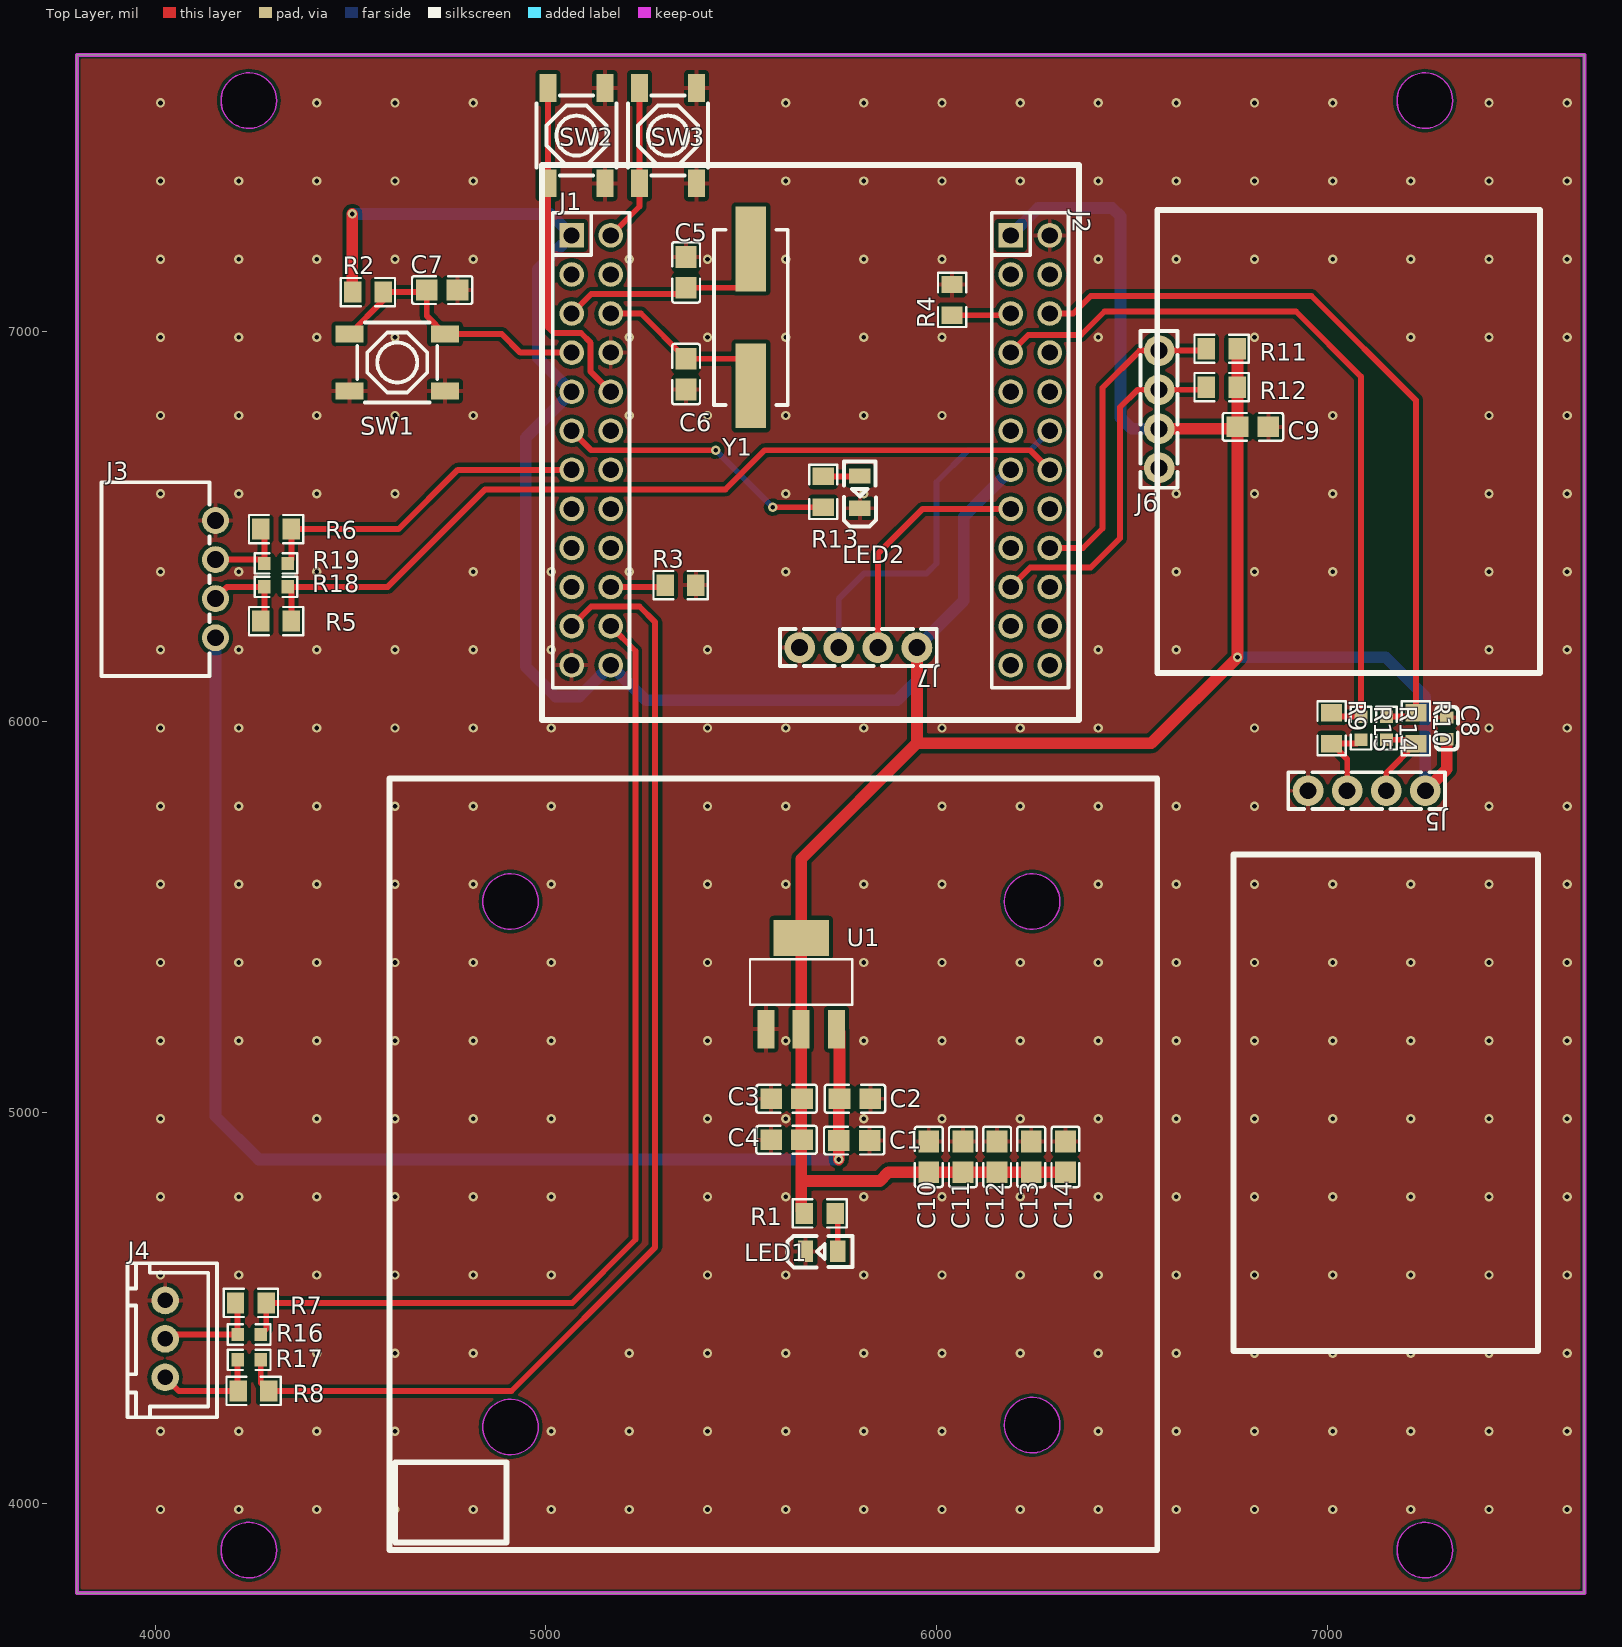
[diagram p0: Top Layer view]
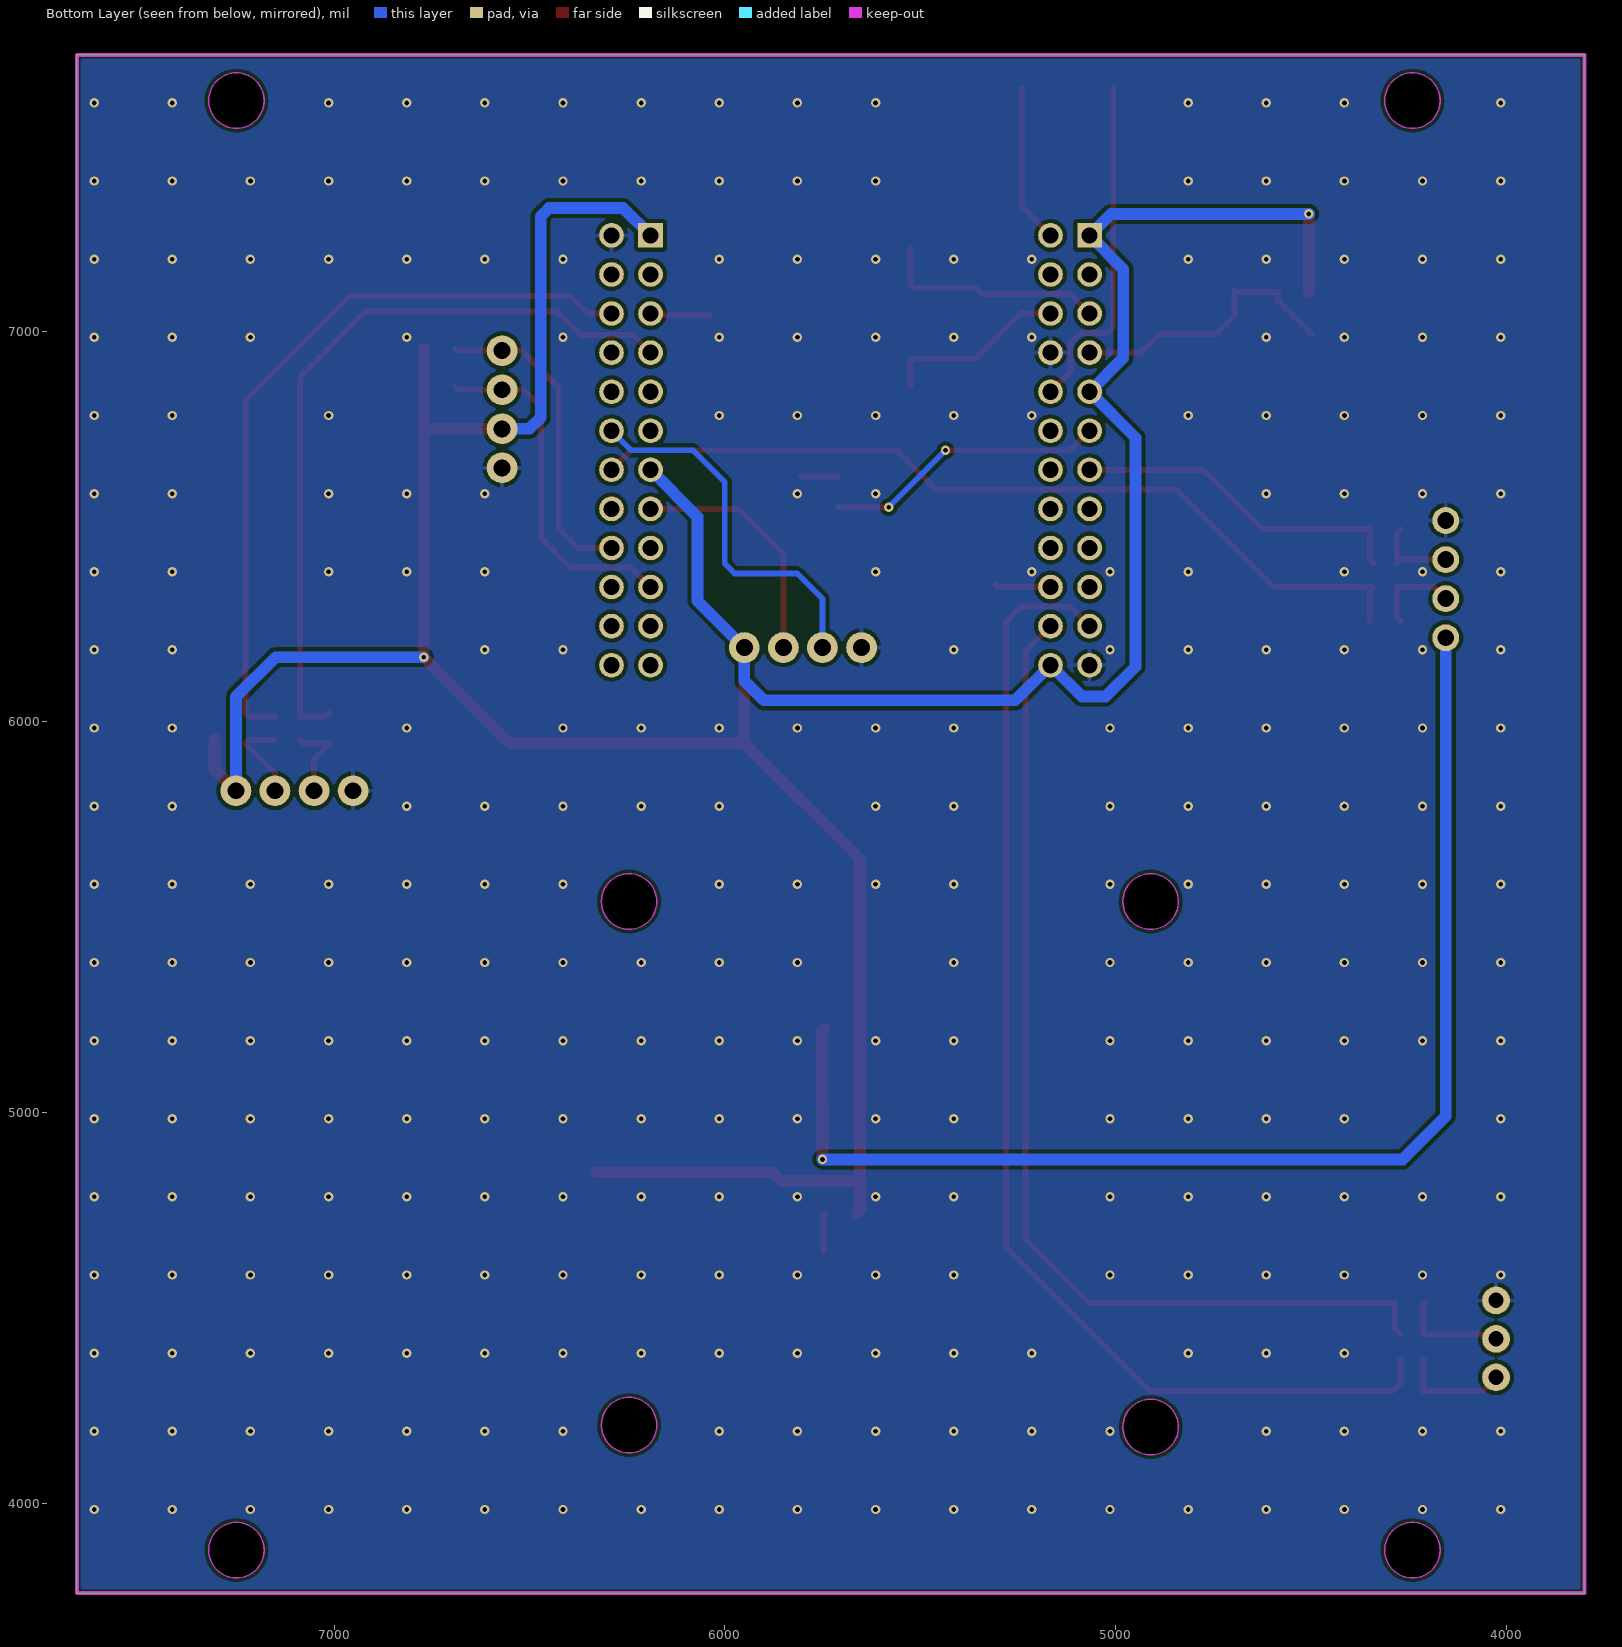
[diagram p1: Bottom Layer view, seen from below]
# Altium PCB MISC52078.pcbdoc
Units mil, origin at the board's own origin, x right, y up, seen from the top; angles counter-clockwise.
Board outline 3858.27 x 3937.01 mil, 2 copper layers (Top Layer, Bottom Layer), stack 2.757 mil thick; 47 components, 30 nets, 155 pads, 300 vias.

## Layer stack, top to bottom
Top Solder Mask Layer: solder mask 0.394, Dk 3.3
Top Layer: signal copper 1.379
Bottom Layer: signal copper 1.378
Bottom Solder Mask Layer: solder mask 0.394, Dk 3.3

## Board outline
3800,7707.01 3800,3770 7658.27,3770 7658.27,7707.01
cut-out: 4981.06,5540 cw(c4910,5540) 4838.94,5540 cw(c4910,5540)
cut-out: 6316.06,5540 cw(c6245,5540) 6173.94,5540 cw(c6245,5540)
cut-out: 6316.06,4200 cw(c6245,4200) 6173.94,4200 cw(c6245,4200)
cut-out: 4981.06,4195 cw(c4910,4195) 4838.94,4195 cw(c4910,4195)
cut-out: 4311.06,3880 cw(c4240,3880) 4168.94,3880 cw(c4240,3880)
cut-out: 4311.06,7590 cw(c4240,7590) 4168.94,7590 cw(c4240,7590)
cut-out: 7321.06,7590 cw(c7250,7590) 7178.94,7590 cw(c7250,7590)
cut-out: 7321.06,3880 cw(c7250,3880) 7178.94,3880 cw(c7250,3880)

## Design rules (kind name [scope] priority, off if disabled: settings)
BoardOutlineClearance Plane_innerPlane_1 [All] p2 off: genericclearance=4 ignorepadtopadclearanceinfootprint=FALSE except(0: Arc-SplitContinuation Track-SplitContinuation SMDPad-SplitContinuation THPad-SplitContinuation Via-SplitContinuation Fill-SplitContinuation Region-SplitContinuation Poly-SplitContinuation Text-SplitContinuation Hole-SplitContinuation; 6: Arc-CutoutEdge Track-CutoutEdge SMDPad-CutoutEdge THPad-CutoutEdge Via-CutoutEdge Text-CutoutEdge; 6.9: Hole-OutlineEdge Hole-CutoutEdge; 10: Poly-OutlineEdge Poly-CutoutEdge; 11.8: Arc-OutlineEdge Track-OutlineEdge SMDPad-OutlineEdge THPad-OutlineEdge Via-OutlineEdge Fill-OutlineEdge Region-OutlineEdge Text-OutlineEdge Fill-CutoutEdge Region-CutoutEdge)
BoardOutlineClearance Copper_copperRegion_1 [All] p4 off: genericclearance=4 ignorepadtopadclearanceinfootprint=FALSE except(0: Arc-SplitContinuation Track-SplitContinuation SMDPad-SplitContinuation THPad-SplitContinuation Via-SplitContinuation Fill-SplitContinuation Region-SplitContinuation Poly-SplitContinuation Text-SplitContinuation Hole-SplitContinuation; 6: Arc-CutoutEdge Track-CutoutEdge SMDPad-CutoutEdge THPad-CutoutEdge Via-CutoutEdge Text-CutoutEdge; 6.9: Hole-OutlineEdge Hole-CutoutEdge; 10: Poly-OutlineEdge Poly-CutoutEdge; 11.8: Arc-OutlineEdge Track-OutlineEdge SMDPad-OutlineEdge THPad-OutlineEdge Via-OutlineEdge Fill-OutlineEdge Region-OutlineEdge Text-OutlineEdge Fill-CutoutEdge Region-CutoutEdge)
BoardOutlineClearance copperThickness1oz_1 [All] p6: genericclearance=4 ignorepadtopadclearanceinfootprint=FALSE except(0: Arc-SplitContinuation Track-SplitContinuation SMDPad-SplitContinuation THPad-SplitContinuation Via-SplitContinuation Fill-SplitContinuation Region-SplitContinuation Poly-SplitContinuation Text-SplitContinuation Hole-SplitContinuation; 6: Arc-CutoutEdge Track-CutoutEdge SMDPad-CutoutEdge THPad-CutoutEdge Via-CutoutEdge Text-CutoutEdge; 6.9: Hole-OutlineEdge Hole-CutoutEdge; 10: Poly-OutlineEdge Poly-CutoutEdge; 11.8: Arc-OutlineEdge Track-OutlineEdge SMDPad-OutlineEdge THPad-OutlineEdge Via-OutlineEdge Fill-OutlineEdge Region-OutlineEdge Text-OutlineEdge Fill-CutoutEdge Region-CutoutEdge)
Clearance Plane_innerPlane [All] p1 off: gap=4 ignorepadtopadclearanceinfootprint=FALSE except(6: SMDPad-Track SMDPad-SMDPad THPad-Track SMDPad-THPad THPad-THPad Track-Via SMDPad-Via THPad-Via Via-Via Fill-SMDPad Region-SMDPad Fill-THPad Region-THPad Fill-Via Region-Via Fill-Fill Fill-Region Region-Region Arc-Track Arc-SMDPad Arc-THPad Arc-Via Fill-Arc Region-Arc Arc-Arc Text-Track SMDPad-Text Text-THPad Text-Via Fill-Text Region-Text Arc-Text Text-Text; 6.9: Hole-Track Hole-SMDPad Hole-THPad Hole-Via Fill-Hole Region-Hole Hole-Arc Hole-Text; 10: Poly-Track Poly-SMDPad Poly-THPad Poly-Via Poly-Fill Poly-Region Poly-Poly Poly-Arc Poly-Text Poly-Hole; 11.8: Fill-Track Region-Track)
Clearance Copper_copperRegion [All] p3 off: gap=4 ignorepadtopadclearanceinfootprint=FALSE except(6: SMDPad-Track SMDPad-SMDPad THPad-Track SMDPad-THPad THPad-THPad Track-Via SMDPad-Via THPad-Via Via-Via Fill-SMDPad Region-SMDPad Fill-THPad Region-THPad Fill-Via Region-Via Fill-Fill Fill-Region Region-Region Arc-Track Arc-SMDPad Arc-THPad Arc-Via Fill-Arc Region-Arc Arc-Arc Text-Track SMDPad-Text Text-THPad Text-Via Fill-Text Region-Text Arc-Text Text-Text; 6.9: Hole-Track Hole-SMDPad Hole-THPad Hole-Via Fill-Hole Region-Hole Hole-Arc Hole-Text; 10: Poly-Track Poly-SMDPad Poly-THPad Poly-Via Poly-Fill Poly-Region Poly-Poly Poly-Arc Poly-Text Poly-Hole; 11.8: Fill-Track Region-Track)
Clearance copperThickness1oz [All] p5: gap=4 ignorepadtopadclearanceinfootprint=FALSE except(6: SMDPad-Track SMDPad-SMDPad THPad-Track SMDPad-THPad THPad-THPad Track-Via SMDPad-Via THPad-Via Via-Via Fill-SMDPad Region-SMDPad Fill-THPad Region-THPad Fill-Via Region-Via Fill-Fill Fill-Region Region-Region Arc-Track Arc-SMDPad Arc-THPad Arc-Via Fill-Arc Region-Arc Arc-Arc Text-Track SMDPad-Text Text-THPad Text-Via Fill-Text Region-Text Arc-Text Text-Text; 6.9: Hole-Track Hole-SMDPad Hole-THPad Hole-Via Fill-Hole Region-Hole Hole-Arc Hole-Text; 10: Poly-Track Poly-SMDPad Poly-THPad Poly-Via Poly-Fill Poly-Region Poly-Poly Poly-Arc Poly-Text Poly-Hole; 11.8: Fill-Track Region-Track)
DiffPairsRouting differentialPair [All] p1: maxlimit=6 minlimit=5 mostfreqgap=6 toplayer_minwidth=5 toplayer_prefwidth=100 toplayer_maxwidth=100 toplayer_mingap=5 toplayer_prefgap=6 toplayer_maxgap=6 bottomlayer_minwidth=5 bottomlayer_prefwidth=100 bottomlayer_maxwidth=100 bottomlayer_mingap=5 bottomlayer_prefgap=6 bottomlayer_maxgap=6 maxuncoupledlength=10
HoleToHoleClearance otherClearance [All] p1: gap=11.8 allowstackedmicrovias=TRUE
Length netLength [All] p1: minlimit=0 maxlimit=0
MatchedLengths netLengthTolerance [All] p1: tolerance=1000
PasteMaskExpansion pasteMaskExpansion [All] p1: expansion=0
PlaneConnect innerPlane [All] p1: planeconnectstyle=Relief reliefexpansion=20 reliefentries=4 reliefconductorwidth=10 reliefairgap=10
PolygonConnect copperRegion [(InNet('GND'))] p1: connectstyle=Relief reliefconductorwidth=10 reliefentries=4 polygonreliefangle="90 Angle" airgapwidth=10 via.connectstyle=Relief via.reliefconductorwidth=10 via.reliefentries=4 via.polygonreliefangle="90 Angle" via.airgapwidth=10
RoutingVias viaSize [All] p1: holewidth=12.01 width=24.02 viastyle="Through Hole" minholewidth=11.81 minwidth=19.68 maxholewidth=248.03 maxwidth=393.7
SolderMaskExpansion solderMaskExpansion [IsVia] p1: expansion=-1000 istentingtop=TRUE
SolderMaskExpansion solderMaskExpansion [All] p2: expansion=2 istentingtop=FALSE
Width copperThickness1oz_2 [All] p1: maxlimit=100 minlimit=5 preferedwidth=10

## Components (designator, comment, footprint, x,y, rotation, side; value= is the part's Value field where it differs from the comment)
C1 "10uF" C0805 5789.54,4928.26 r0 top
C2 "0.1uF" C0805 5791.42,5035.2 r0 top
C3 "10uF" C0805 5616.42,5035.2 r0 top
C4 "0.1uF" C0805 5616.42,4930.2 r0 top
C5 "20pF" C0805 5359.24,7150.22 r270 top
C6 "20pF" C0805 5359.24,6890 r90 top
C7 "10uF" C0805 4735,7105 r0 top
C8 "0.1uF" C0603 7306.26,5983.34 r270 top
C9 "0.1uF" C0805 6810,6755 r0 top
C10 "0.1uF" C0805 5980.2,4886.53 r90 top
C11 "0.1uF" C0805 6067.7,4886.53 r90 top
C12 "0.1uF" C0805 6155.2,4886.53 r90 top
C13 "0.1uF" C0805 6242.7,4886.53 r90 top
C14 "0.1uF" C0805 6330.2,4886.53 r90 top
J1 "PM254-2-12-Z-8.5" HDR-TH_24P-P2.54-V-F-R2-C12-S2.54-2 5116.37,6695 r270 top
J2 "PM254-2-12-Z-8.5" HDR-TH_24P-P2.54-V-F-R2-C12-S2.54-2 6240,6695 r270 top
J3 "XH-4AW" CONN-TH_XH-4AW 4154.72,6365.22 r270 top
J4 "XH-3A" CONN-TH_XH-3A 4026.06,4420.68 r270 top
J5 "" CONN-TH_4P-P2.54-L10.2-W2.5 7101.26,5823.64 r180 top
J6 "" CONN-TH_4P-P2.54-L10.2-W2.5 6570,6800 r90 top
J7 "" CONN-TH_4P-P2.54-L10.2-W2.5 5800,6190 r180 top
LED1 "KT-0805W" LED0805-R-RD 5706.21,4644.51 r0 top
LED2 "" LED0805-R-RD 5803.84,6587.94 r90 top
R1 "510" R0805 5701.13,4741.93 r0 top
R2 "10K" R0805 4545,7100 r180 top
R3 "10K" R0805 5345.01,6349.76 r0 top
R4 "10K" R0805 6040,7080 r90 top
R5 "22R" R0805 4309.72,6257.67 r180 top
R6 "22R" R0805 4309.72,6493.27 r180 top
R7 "22R" R0805 4245.43,4512.7 r180 top
R8 "22R" R0805 4252.16,4287.39 r180 top
R9 "22R" R0805 7011.26,5983.64 r270 top
R10 "22R" R0805 7227.03,5983.64 r270 top
R11 "4.7K" R0805 6730,6955 r0 top
R12 "4.7K" R0805 6730,6856.57 r0 top
R13 "510" R0805 5710.11,6588.65 r90 top
R14 "0R" R0603 7151.74,5983.64 r270 top
R15 "0R" R0603 7086.55,5983.64 r270 top
R16 "0R" R0603 4241.06,4432.07 r180 top
R17 "0R" R0603 4241.06,4367.07 r180 top
R18 "0R" R0603 4309.72,6345.47 r180 top
R19 "0R" R0603 4309.72,6405.47 r180 top
SW1 "TS-1087S" SW-SMD_L5.2-W5.2-P3.70-LS6.4 4620,6919.76 r0 top
SW2 "TS-1087S" SW-SMD_L5.2-W5.2-P3.70-LS6.4 5078.51,7500.38 r90 top
SW3 "TS-1087S" SW-SMD_L5.2-W5.2-P3.70-LS6.4 5312.92,7500.38 r90 top
U1 "AMS1117-3.3" SOT-223-3_L6.5-W3.4-P2.30-LS7.0-BR 5653.85,5330.28 r270 top
Y1 "8MHz" CRYSTAL-SMD_L11.5-W4.8-LS12.7 5525,7035 r90 top

## Footprints (in the part's own frame and the unit in brackets; to place one, negate y for a bottom-side part, rotate by r counter-clockwise, add the part's x,y. Pads: shape width x height; smd on the part's side, far side on the other; paste and mask are expansions set on the pad)
C0603 [mm]
  rect 0.8x0.9 smd: 1(-0.7,0) 2(0.7,0)
  silkscreen extent -1.41,-0.71 1.39,0.72
C0805 [mm]
  rect 1.41x1.35 smd paste-100 mask+0.051: 1(-1,0) 2(1,0)
  silkscreen extent -1.96,-0.9 1.96,0.9
CONN-TH_4P-P2.54-L10.2-W2.5 [mm]
  round 2 hole 1.1 paste+0 mask+0.05: 1(-3.81,0) 2(-1.27,0) 3(1.27,0) 4(3.81,0)
  silkscreen extent -5.1,-1.2 5.1,1.2
CONN-TH_XH-3A [mm]
  round 1.8 hole 1 paste+0 mask+0.05: 1(-2.5,0) 2(0,0) 3(2.5,0)
  silkscreen extent -4.92,-2.44 5.09,3.38
CONN-TH_XH-4AW [mm]
  round 1.75 hole 1.1 paste+0 mask+0.05: 1(-3.81,0) 2(-1.27,0) 3(1.27,0) 4(3.81,0)
  silkscreen extent -6.3,-7.4 6.3,-0.4
CRYSTAL-SMD_L11.5-W4.8-LS12.7 [mm]
  rect 5.5x2 smd: 1(-4.45,0) 2(4.45,0)
  silkscreen extent -5.7,-2.4 5.7,2.4
HDR-TH_24P-P2.54-V-F-R2-C12-S2.54-2 [mm]
  rect 1.6x1.6 hole 1.05: 1(-13.97,-1.27)
  round 1.6 hole 1.05: 2(-13.97,1.27) 3(-11.43,-1.27) 4(-11.43,1.27) 5(-8.89,-1.27) 6(-8.89,1.27) 7(-6.35,-1.27) 8(-6.35,1.27) 9(-3.81,-1.27) 10(-3.81,1.27) 11(-1.27,-1.27) 12(-1.27,1.27) 13(1.27,-1.27) 14(1.27,1.27) 15(3.81,-1.27) 16(3.81,1.27) 17(6.35,-1.27) 18(6.35,1.27) 19(8.89,-1.27) 20(8.89,1.27) 21(11.43,-1.27) 22(11.43,1.27) 23(13.97,-1.27) 24(13.97,1.27)
  silkscreen extent -15.44,-2.5 15.44,2.5
LED0805-R-RD [mm]
  rect 1x1.4 smd: 1(1.05,0) 2(-1.05,0)
  silkscreen extent -2.22,-1.04 1.99,1.01
R0603 [mil]
  rect 31.75x34.02 smd paste-3937.01 mask+2: 1(-29.66,0) 2(29.66,0)
  silkscreen extent -55,-26 55,26
R0805 [mm]
  rect 1.133x1.377 smd paste-100 mask+0.051: 1(-1,0) 2(1,0)
  silkscreen extent -1.76,-0.92 1.76,0.92
SOT-223-3_L6.5-W3.4-P2.30-LS7.0-BR [mm]
  rect 2.5x1.1 smd: 1(2.97,-2.3) 2(2.97,0) 3(2.97,2.3)
  rect 2.34x3.6 smd: 4(-2.97,0)
  silkscreen extent -1.57,-3.33 1.37,3.33
SW-SMD_L5.2-W5.2-P3.70-LS6.4 [mm]
  rect 1.8x1.1 smd: 1(-3.1,1.85) 1(3.1,1.85) 2(-3.1,-1.85) 2(3.1,-1.85)
  silkscreen extent -2.6,-2.6 2.6,2.6

## Via types
v1: diameter 24.02, hole 12, Top Layer to Bottom Layer, 300 vias

## Nets (pads, with @x,y where several pads share a name; then routed paths per layer and width w, separated by ;. In a path a pad name is that pad's centre, name@x,y a point inside that pad or via, vN(x,y) a via of type N, cw(c..) or ccw(c..) an arc to the next point about the centre after c; other vN are vias at no path point)
$1N51: LED1.1 R1.2 | length 100.3
  Top Layer w15: R1.2 5747.56,4734.87 LED1.1
$1N94: LED2.1 R13.2 | length 94.3
  Top Layer w15: R13.2 5802.57,6628.02 LED2.1
$1N2341: J5.3 R9.2 R15.2 | length 216.5
  Top Layer w15: J5.3 7051.26,5904.27 R9.2 7076.84,5944.27 R15.2
$1N2343: J5.2 R10.2 R14.2 | length 231.3
  Top Layer w15: J5.2 7151.26,5868.51 R10.2 7217.32,5953.98 R14.2
$1N2365: J1.12
$1N2372: J4.3 R8.2 R17.2 | length 281.4
  Top Layer w15: J4.3 4060.92,4287.39 R8.2 4211.4,4288.78 R17.2
$1N2373: J4.2 R7.2 R16.2 | length 272.9
  Top Layer w15: J4.2 4037.44,4432.07 R16.2 4211.4,4507.36 R7.2
$1N2382: J3.2 R6.2 R19.2 | length 221.2
  Top Layer w15: J3.2 4270.31,6415.22 R19.2 4280.06,6483.56 R6.2
$1N2384: J3.3 R5.2 R18.2 | length 229.7
  Top Layer w15: J3.3 4184.97,6345.47 R18.2 4280.06,6267.38 R5.2
+3.3V: C3.2 C4.2 C8.2 C9.1 C10.1 C11.1 C12.1 C13.1 C14.1 J1.1 J1.9 J1.24 J2.1 J2.13 J5.1 J6.2 J7.1 R1.1 R2.2 R11.2 R12.2 U1.2 U1.4 | length 9798.6
  Top Layer w30: v1(4505,7300) 4505,7100.63 R2.2 ; R1.1 5653.85,4749.85 5653.85,4824.62 ; J7.1 5950,5945 ; C14.1 C13.1 C12.1 C11.1 C10.1 5877.16,4847.16 5854.62,4824.62 5653.85,4824.62 ; J6.2 6765.63,6750 C9.1 ; R11.2 6770.63,6953.74 C9.1 ; J5.1 7306.26,5878.64 C8.2 ; 5653.85,4824.62 U1.2 U1.4 5653.85,5648.85 5950,5945 ; 5950,5945 6550,5945 v1(6770.63,6165.63) C9.1
  Bottom Layer w30: v1(4505,7300) 5011.37,7300 J1.1 4980,7158.63 4980,6931.37 J1.9 4948.79,6727.42 4948.79,6141.21 5025,6065 5086.37,6065 J1.24 5256.37,6055 5900,6055 5950,6105 J7.1 6070,6310 6070,6525 J2.13 ; J2.1 6260,7315 6450,7315 6471.21,7293.79 6471.21,6778.79 6500,6750 J6.2 ; v1(6770.63,6165.63) 7149.37,6165.63 7251.26,6063.74 J5.1
+5V: C1.1 C2.1 J3.4 U1.3 | length 3203.3
  Top Layer w30: U1.3 5752.05,5205.7 C2.1 5750,5033.15 v1(5750,4880)
  Bottom Layer w30: J3.4 4154.72,4990.28 4265,4880 v1(5750,4880)
BOOT0: J2.5 R4.1 | length 151.8
  Top Layer w15: R4.1 6185.63,7040.63 J2.5
BOOT1: J1.20 R3.1 | length 141.2
  Top Layer w15: J1.20 5300.88,6345 R3.1
GND: C1.2 C2.2 C3.1 C4.1 C5.1 C6.1 C7.2 C8.1 C9.2 C10.2 C11.2 C12.2 C13.2 C14.2 J1.8 J1.23 J2.2 J3.1 J4.1 J5.4 J6.1 J7.4 LED1.2 LED2.2 R3.2 R4.2 SW1.2 SW2.2 SW3.2 U1.1
  other v1: 4014.1,3984.1 4214.1,3984.1 4414.1,3984.1 4614.1,3984.1 4814.1,3984.1 5014.1,3984.1 5214.1,3984.1 5414.1,3984.1 5614.1,3984.1 5814.1,3984.1 6014.1,3984.1 6214.1,3984.1 6414.1,3984.1 6614.1,3984.1 6814.1,3984.1 7014.1,3984.1 7214.1,3984.1 7414.1,3984.1 7614.1,3984.1 4014.1,4184.1 4214.1,4184.1 4414.1,4184.1 4614.1,4184.1 5014.1,4184.1 5214.1,4184.1 5414.1,4184.1 5614.1,4184.1 5814.1,4184.1 6014.1,4184.1 6414.1,4184.1 6614.1,4184.1 6814.1,4184.1 7014.1,4184.1 7214.1,4184.1 7414.1,4184.1 7614.1,4184.1 4414.1,4384.1 4614.1,4384.1 4814.1,4384.1 5214.1,4384.1 5414.1,4384.1 5614.1,4384.1 5814.1,4384.1 6014.1,4384.1 6214.1,4384.1 6414.1,4384.1 6614.1,4384.1 6814.1,4384.1 7014.1,4384.1 7214.1,4384.1 7414.1,4384.1 7614.1,4384.1 4014.1,4584.1 4214.1,4584.1 4414.1,4584.1 4614.1,4584.1 4814.1,4584.1 5014.1,4584.1 5414.1,4584.1 5614.1,4584.1 5814.1,4584.1 6014.1,4584.1 6214.1,4584.1 6414.1,4584.1 6614.1,4584.1 6814.1,4584.1 7014.1,4584.1 7214.1,4584.1 7414.1,4584.1 7614.1,4584.1 4014.1,4784.1 4214.1,4784.1 4414.1,4784.1 4614.1,4784.1 4814.1,4784.1 5014.1,4784.1 5414.1,4784.1 5614.1,4784.1 5814.1,4784.1 6014.1,4784.1 6214.1,4784.1 6414.1,4784.1 6614.1,4784.1 6814.1,4784.1 7014.1,4784.1 7214.1,4784.1 7414.1,4784.1 7614.1,4784.1 4014.1,4984.1 4414.1,4984.1 4614.1,4984.1 4814.1,4984.1 5014.1,4984.1 5414.1,4984.1 5614.1,4984.1 5814.1,4984.1 6014.1,4984.1 6214.1,4984.1 6414.1,4984.1 6614.1,4984.1 6814.1,4984.1 7014.1,4984.1 7214.1,4984.1 7414.1,4984.1 7614.1,4984.1 4014.1,5184.1 4214.1,5184.1 4414.1,5184.1 4614.1,5184.1 4814.1,5184.1 5014.1,5184.1 5414.1,5184.1 5614.1,5184.1 5814.1,5184.1 6014.1,5184.1 6214.1,5184.1 6414.1,5184.1 6614.1,5184.1 6814.1,5184.1 7014.1,5184.1 7214.1,5184.1 7414.1,5184.1 7614.1,5184.1 4014.1,5384.1 4214.1,5384.1 4414.1,5384.1 4614.1,5384.1 4814.1,5384.1 5014.1,5384.1 5414.1,5384.1 5814.1,5384.1 6014.1,5384.1 6214.1,5384.1 6414.1,5384.1 6614.1,5384.1 6814.1,5384.1 7014.1,5384.1 7214.1,5384.1 7414.1,5384.1 7614.1,5384.1 4014.1,5584.1 4214.1,5584.1 4414.1,5584.1 4614.1,5584.1 4814.1,5584.1 5014.1,5584.1 5414.1,5584.1 5614.1,5584.1 5814.1,5584.1 6014.1,5584.1 6414.1,5584.1 6614.1,5584.1 6814.1,5584.1 7014.1,5584.1 7214.1,5584.1 7414.1,5584.1 7614.1,5584.1 4014.1,5784.1 4214.1,5784.1 4414.1,5784.1 4614.1,5784.1 4814.1,5784.1 5014.1,5784.1 5414.1,5784.1 5614.1,5784.1 6014.1,5784.1 6214.1,5784.1 6414.1,5784.1 6614.1,5784.1 6814.1,5784.1 7414.1,5784.1 7614.1,5784.1 4014.1,5984.1 4214.1,5984.1 4414.1,5984.1 4614.1,5984.1 4814.1,5984.1 5014.1,5984.1 5414.1,5984.1 5614.1,5984.1 5814.1,5984.1 6014.1,5984.1 6214.1,5984.1 6414.1,5984.1 6814.1,5984.1 7414.1,5984.1 7614.1,5984.1 4014.1,6184.1 4214.1,6184.1 4414.1,6184.1 4614.1,6184.1 4814.1,6184.1 5014.1,6184.1 5414.1,6184.1 6414.1,6184.1 6614.1,6184.1 7414.1,6184.1 7614.1,6184.1 4014.1,6384.1 4214.1,6384.1 4414.1,6384.1 4814.1,6384.1 5014.1,6384.1 5214.1,6384.1 5614.1,6384.1 6614.1,6384.1 6814.1,6384.1 7014.1,6384.1 7414.1,6384.1 7614.1,6384.1 4014.1,6584.1 4214.1,6584.1 4414.1,6584.1 4614.1,6584.1 5614.1,6584.1 5814.1,6584.1 6614.1,6584.1 6814.1,6584.1 7014.1,6584.1 7414.1,6584.1 7614.1,6584.1 4014.1,6784.1 4214.1,6784.1 4414.1,6784.1 4614.1,6784.1 4814.1,6784.1 5214.1,6784.1 5414.1,6784.1 5614.1,6784.1 5814.1,6784.1 6014.1,6784.1 7014.1,6784.1 7414.1,6784.1 7614.1,6784.1 4014.1,6984.1 4214.1,6984.1 4414.1,6984.1 4614.1,6984.1 5214.1,6984.1 5414.1,6984.1 5614.1,6984.1 5814.1,6984.1 6014.1,6984.1 6414.1,6984.1 6814.1,6984.1 7214.1,6984.1 7414.1,6984.1 7614.1,6984.1 4014.1,7184.1 4214.1,7184.1 4414.1,7184.1 4614.1,7184.1 4814.1,7184.1 5214.1,7184.1 5414.1,7184.1 5614.1,7184.1 5814.1,7184.1 6014.1,7184.1 6414.1,7184.1 6614.1,7184.1 6814.1,7184.1 7014.1,7184.1 7214.1,7184.1 7414.1,7184.1 7614.1,7184.1 4014.1,7384.1 4214.1,7384.1 4414.1,7384.1 4614.1,7384.1 4814.1,7384.1 5614.1,7384.1 5814.1,7384.1 6014.1,7384.1 6214.1,7384.1 6414.1,7384.1 6614.1,7384.1 6814.1,7384.1 7014.1,7384.1 7214.1,7384.1 7414.1,7384.1 7614.1,7384.1 4014.1,7584.1 4414.1,7584.1 4614.1,7584.1 4814.1,7584.1 5614.1,7584.1 5814.1,7584.1 6014.1,7584.1 6214.1,7584.1 6414.1,7584.1 6614.1,7584.1 6814.1,7584.1 7014.1,7584.1 7414.1,7584.1 7614.1,7584.1
I2C1_SCL: J2.19 J6.3 R12.1 | length 908.8
  Top Layer w15: J2.19 6240,6395 6395,6395 6470,6470 6470,6805 6515,6850 J6.3 6684.06,6850 R12.1
I2C1_SDA: J2.18 J6.4 R11.1 | length 822.8
  Top Layer w15: J2.18 6375,6445 6425,6495 6425,6855 6520,6950 J6.4 6685.63,6950 R11.1
NRST: C7.1 J1.7 R2.1 SW1.1 | length 732.2
  Top Layer w15: SW1.1@4497.95,6992.6 4584.37,7079.02 R2.1 4690.63,7100 C7.1 4695.63,7039.02 4742.05,6992.6 4887.4,6992.6 4935,6945 J1.7
OSC_IN: C5.2 J1.5 Y1.2 | length 579.9
  Top Layer w15: J1.5 5116.37,7095 5343.4,7095 C5.2 5515.85,7110.85 5525,7120 Y1.2
OSC_OUT: C6.2 J1.6 Y1.1 | length 476.1
  Top Layer w15: J1.6 5243.61,7045 C6.2 5525,6929.37 Y1.1
PA0: J1.10 SW2.1 | length 885
  Top Layer w15: SW2.1@5005.67,7622.43 5005.67,7378.33 5005.67,7009.33 5020,6995 5090,6995 5115,6970 5115,6896.37 J1.10
PA1: J1.11 R13.1 | length 724.8
  Top Layer w15: J1.11 5116.37,6695 v1(5435,6695) ; v1@5579.78,6550.22 v1(5580.72,6549.28) R13.1
  Bottom Layer w15: v1(5435,6695) v1@5579.78,6550.22
PC13: J1.2 SW3.1 | length 408
  Top Layer w15: J1.2 5240.08,7318.72 5240.08,7378.33 SW3.1@5240.08,7622.43
SWCLK: J2.12 J7.3 | length 965.4
  Bottom Layer w15: J7.3 5750,6315 5815,6380 5975,6380 6000,6405 6000,6613.73 6081.27,6695 6240,6695 J2.12
SWDIO: J2.15 J7.2 | length 627.6
  Top Layer w15: J7.2 5850,6430 5965,6545 J2.15
USART1_RX: J2.6 R10.1 R14.1 | length 1945.5
  Top Layer w15: J2.6 6350,7045 6395,7090 6960,7090 7227.03,6822.97 R10.1 7217.32,6013.3 R14.1
USART1_TX: J2.7 R9.1 R15.1 | length 1958.5
  Top Layer w15: J2.7 6235,6990 6370,6990 6430,7050 6920,7050 7086.55,6883.45 R15.1 7020.97,6013.3 R9.1
USART2_RX: J1.13 R6.1 R19.1 | length 871.9
  Top Layer w15: R19.1 4349.09,6415.18 R6.1 4623.27,6493.27 4775,6645 J1.13
USART2_TX: J2.14 R5.1 R18.1 | length 2207.9
  Top Layer w15: R5.1 4349.09,6335.76 R18.1 4595.47,6345.47 4845,6595 5460,6595 5560,6695 6240,6695 J2.14
USART3_RX: J1.22 R7.1 R16.1 | length 2695.2
  Top Layer w15: R16.1 4284.8,4446.15 R7.1 5067.7,4512.7 5230,4675 5230,6181.37 J1.22
USART3_TX: J1.21 R8.1 R17.1 | length 3079.9
  Top Layer w15: R17.1 4270.72,4308.2 R8.1 4912.39,4287.39 5280,4655 5280,6255 5240,6295 5116.37,6295 J1.21
pads on no net: J1.3 J1.4 J1.14 J1.15 J1.16 J1.17 J1.18 J1.19 J2.3 J2.4 J2.8 J2.9 J2.10 J2.11 J2.16 J2.17 J2.20 J2.21 J2.22 J2.23 J2.24

## Polygon pours and split planes (outlines as drawn)
GND on Top Layer (solid, remove dead copper, pour order 0): 3485,7905 3485,3750 8125,3750 8125,7905
GND on Bottom Layer (solid, remove dead copper, pour order 2): 3000,8475 3000,3000 8510,3000 8510,8475

## Keep-outs
Board Outline Layer:
  region: 4981.06,5540 cw(c4910,5540) 4838.94,5540 cw(c4910,5540)
  circle w0.1: c4910,5540 r71.06
  region: 4981.06,5540 4980.67,5532.57 4979.51,5525.23 4977.59,5518.04 4974.92,5511.1 4971.54,5504.47 4967.49,5498.23 4962.81,5492.45 4957.55,5487.19 4951.77,5482.51 4945.53,5478.46 4938.9,5475.08 4931.96,5472.41 4924.77,5470.49 4917.43,5469.33 4910,5468.94 4902.57,5469.33 4895.23,5470.49 4888.04,5472.41 4881.1,5475.08 4874.47,5478.46 4868.23,5482.51 4862.45,5487.19 4857.19,5492.45 4852.51,5498.23 4848.46,5504.47 4845.08,5511.1 4842.41,5518.04 4840.49,5525.23 4839.33,5532.57 4838.94,5540 4839.33,5547.43 4840.49,5554.77 4842.41,5561.96 4845.08,5568.9 4848.46,5575.53 4852.51,5581.77 4857.19,5587.55 4862.45,5592.81 4868.23,5597.49 4874.47,5601.54 4881.1,5604.92 4888.04,5607.59 4895.23,5609.51 4902.57,5610.67 4910,5611.06 4917.43,5610.67 4924.77,5609.51 4931.96,5607.59 4938.9,5604.92 4945.53,5601.54 4951.77,5597.49 4957.55,5592.81 4962.81,5587.55 4967.49,5581.77 4971.54,5575.53 4974.92,5568.9 4977.59,5561.96 4979.51,5554.77 4980.67,5547.43
  region: 6316.06,5540 cw(c6245,5540) 6173.94,5540 cw(c6245,5540)
  circle w0.1: c6245,5540 r71.06
  region: 6316.06,5540 6315.67,5532.57 6314.51,5525.23 6312.59,5518.04 6309.92,5511.1 6306.54,5504.47 6302.49,5498.23 6297.81,5492.45 6292.55,5487.19 6286.77,5482.51 6280.53,5478.46 6273.9,5475.08 6266.96,5472.41 6259.77,5470.49 6252.43,5469.33 6245,5468.94 6237.57,5469.33 6230.23,5470.49 6223.04,5472.41 6216.1,5475.08 6209.47,5478.46 6203.23,5482.51 6197.45,5487.19 6192.19,5492.45 6187.51,5498.23 6183.46,5504.47 6180.08,5511.1 6177.41,5518.04 6175.49,5525.23 6174.33,5532.57 6173.94,5540 6174.33,5547.43 6175.49,5554.77 6177.41,5561.96 6180.08,5568.9 6183.46,5575.53 6187.51,5581.77 6192.19,5587.55 6197.45,5592.81 6203.23,5597.49 6209.47,5601.54 6216.1,5604.92 6223.04,5607.59 6230.23,5609.51 6237.57,5610.67 6245,5611.06 6252.43,5610.67 6259.77,5609.51 6266.96,5607.59 6273.9,5604.92 6280.53,5601.54 6286.77,5597.49 6292.55,5592.81 6297.81,5587.55 6302.49,5581.77 6306.54,5575.53 6309.92,5568.9 6312.59,5561.96 6314.51,5554.77 6315.67,5547.43
  region: 6316.06,4200 cw(c6245,4200) 6173.94,4200 cw(c6245,4200)
  circle w0.1: c6245,4200 r71.06
  region: 6316.06,4200 6315.67,4192.57 6314.51,4185.23 6312.59,4178.04 6309.92,4171.1 6306.54,4164.47 6302.49,4158.23 6297.81,4152.45 6292.55,4147.19 6286.77,4142.51 6280.53,4138.46 6273.9,4135.08 6266.96,4132.41 6259.77,4130.49 6252.43,4129.33 6245,4128.94 6237.57,4129.33 6230.23,4130.49 6223.04,4132.41 6216.1,4135.08 6209.47,4138.46 6203.23,4142.51 6197.45,4147.19 6192.19,4152.45 6187.51,4158.23 6183.46,4164.47 6180.08,4171.1 6177.41,4178.04 6175.49,4185.23 6174.33,4192.57 6173.94,4200 6174.33,4207.43 6175.49,4214.77 6177.41,4221.96 6180.08,4228.9 6183.46,4235.53 6187.51,4241.77 6192.19,4247.55 6197.45,4252.81 6203.23,4257.49 6209.47,4261.54 6216.1,4264.92 6223.04,4267.59 6230.23,4269.51 6237.57,4270.67 6245,4271.06 6252.43,4270.67 6259.77,4269.51 6266.96,4267.59 6273.9,4264.92 6280.53,4261.54 6286.77,4257.49 6292.55,4252.81 6297.81,4247.55 6302.49,4241.77 6306.54,4235.53 6309.92,4228.9 6312.59,4221.96 6314.51,4214.77 6315.67,4207.43
  region: 4981.06,4195 cw(c4910,4195) 4838.94,4195 cw(c4910,4195)
  circle w0.1: c4910,4195 r71.06
  region: 4981.06,4195 4980.67,4187.57 4979.51,4180.23 4977.59,4173.04 4974.92,4166.1 4971.54,4159.47 4967.49,4153.23 4962.81,4147.45 4957.55,4142.19 4951.77,4137.51 4945.53,4133.46 4938.9,4130.08 4931.96,4127.41 4924.77,4125.49 4917.43,4124.33 4910,4123.94 4902.57,4124.33 4895.23,4125.49 4888.04,4127.41 4881.1,4130.08 4874.47,4133.46 4868.23,4137.51 4862.45,4142.19 4857.19,4147.45 4852.51,4153.23 4848.46,4159.47 4845.08,4166.1 4842.41,4173.04 4840.49,4180.23 4839.33,4187.57 4838.94,4195 4839.33,4202.43 4840.49,4209.77 4842.41,4216.96 4845.08,4223.9 4848.46,4230.53 4852.51,4236.77 4857.19,4242.55 4862.45,4247.81 4868.23,4252.49 4874.47,4256.54 4881.1,4259.92 4888.04,4262.59 4895.23,4264.51 4902.57,4265.67 4910,4266.06 4917.43,4265.67 4924.77,4264.51 4931.96,4262.59 4938.9,4259.92 4945.53,4256.54 4951.77,4252.49 4957.55,4247.81 4962.81,4242.55 4967.49,4236.77 4971.54,4230.53 4974.92,4223.9 4977.59,4216.96 4979.51,4209.77 4980.67,4202.43
  region: 4311.06,3880 cw(c4240,3880) 4168.94,3880 cw(c4240,3880)
  circle w0.1: c4240,3880 r71.06
  region: 4311.06,3880 4310.67,3872.57 4309.51,3865.23 4307.59,3858.04 4304.92,3851.1 4301.54,3844.47 4297.49,3838.23 4292.81,3832.45 4287.55,3827.19 4281.77,3822.51 4275.53,3818.46 4268.9,3815.08 4261.96,3812.41 4254.77,3810.49 4247.43,3809.33 4240,3808.94 4232.57,3809.33 4225.23,3810.49 4218.04,3812.41 4211.1,3815.08 4204.47,3818.46 4198.23,3822.51 4192.45,3827.19 4187.19,3832.45 4182.51,3838.23 4178.46,3844.47 4175.08,3851.1 4172.41,3858.04 4170.49,3865.23 4169.33,3872.57 4168.94,3880 4169.33,3887.43 4170.49,3894.77 4172.41,3901.96 4175.08,3908.9 4178.46,3915.53 4182.51,3921.77 4187.19,3927.55 4192.45,3932.81 4198.23,3937.49 4204.47,3941.54 4211.1,3944.92 4218.04,3947.59 4225.23,3949.51 4232.57,3950.67 4240,3951.06 4247.43,3950.67 4254.77,3949.51 4261.96,3947.59 4268.9,3944.92 4275.53,3941.54 4281.77,3937.49 4287.55,3932.81 4292.81,3927.55 4297.49,3921.77 4301.54,3915.53 4304.92,3908.9 4307.59,3901.96 4309.51,3894.77 4310.67,3887.43
  region: 4311.06,7590 cw(c4240,7590) 4168.94,7590 cw(c4240,7590)
  circle w0.1: c4240,7590 r71.06
  region: 4311.06,7590 4310.67,7582.57 4309.51,7575.23 4307.59,7568.04 4304.92,7561.1 4301.54,7554.47 4297.49,7548.23 4292.81,7542.45 4287.55,7537.19 4281.77,7532.51 4275.53,7528.46 4268.9,7525.08 4261.96,7522.41 4254.77,7520.49 4247.43,7519.33 4240,7518.94 4232.57,7519.33 4225.23,7520.49 4218.04,7522.41 4211.1,7525.08 4204.47,7528.46 4198.23,7532.51 4192.45,7537.19 4187.19,7542.45 4182.51,7548.23 4178.46,7554.47 4175.08,7561.1 4172.41,7568.04 4170.49,7575.23 4169.33,7582.57 4168.94,7590 4169.33,7597.43 4170.49,7604.77 4172.41,7611.96 4175.08,7618.9 4178.46,7625.53 4182.51,7631.77 4187.19,7637.55 4192.45,7642.81 4198.23,7647.49 4204.47,7651.54 4211.1,7654.92 4218.04,7657.59 4225.23,7659.51 4232.57,7660.67 4240,7661.06 4247.43,7660.67 4254.77,7659.51 4261.96,7657.59 4268.9,7654.92 4275.53,7651.54 4281.77,7647.49 4287.55,7642.81 4292.81,7637.55 4297.49,7631.77 4301.54,7625.53 4304.92,7618.9 4307.59,7611.96 4309.51,7604.77 4310.67,7597.43
  region: 7321.06,7590 cw(c7250,7590) 7178.94,7590 cw(c7250,7590)
  circle w0.1: c7250,7590 r71.06
  region: 7321.06,7590 7320.67,7582.57 7319.51,7575.23 7317.59,7568.04 7314.92,7561.1 7311.54,7554.47 7307.49,7548.23 7302.81,7542.45 7297.55,7537.19 7291.77,7532.51 7285.53,7528.46 7278.9,7525.08 7271.96,7522.41 7264.77,7520.49 7257.43,7519.33 7250,7518.94 7242.57,7519.33 7235.23,7520.49 7228.04,7522.41 7221.1,7525.08 7214.47,7528.46 7208.23,7532.51 7202.45,7537.19 7197.19,7542.45 7192.51,7548.23 7188.46,7554.47 7185.08,7561.1 7182.41,7568.04 7180.49,7575.23 7179.33,7582.57 7178.94,7590 7179.33,7597.43 7180.49,7604.77 7182.41,7611.96 7185.08,7618.9 7188.46,7625.53 7192.51,7631.77 7197.19,7637.55 7202.45,7642.81 7208.23,7647.49 7214.47,7651.54 7221.1,7654.92 7228.04,7657.59 7235.23,7659.51 7242.57,7660.67 7250,7661.06 7257.43,7660.67 7264.77,7659.51 7271.96,7657.59 7278.9,7654.92 7285.53,7651.54 7291.77,7647.49 7297.55,7642.81 7302.81,7637.55 7307.49,7631.77 7311.54,7625.53 7314.92,7618.9 7317.59,7611.96 7319.51,7604.77 7320.67,7597.43
  region: 7321.06,3880 cw(c7250,3880) 7178.94,3880 cw(c7250,3880)
  circle w0.1: c7250,3880 r71.06
  region: 7321.06,3880 7320.67,3872.57 7319.51,3865.23 7317.59,3858.04 7314.92,3851.1 7311.54,3844.47 7307.49,3838.23 7302.81,3832.45 7297.55,3827.19 7291.77,3822.51 7285.53,3818.46 7278.9,3815.08 7271.96,3812.41 7264.77,3810.49 7257.43,3809.33 7250,3808.94 7242.57,3809.33 7235.23,3810.49 7228.04,3812.41 7221.1,3815.08 7214.47,3818.46 7208.23,3822.51 7202.45,3827.19 7197.19,3832.45 7192.51,3838.23 7188.46,3844.47 7185.08,3851.1 7182.41,3858.04 7180.49,3865.23 7179.33,3872.57 7178.94,3880 7179.33,3887.43 7180.49,3894.77 7182.41,3901.96 7185.08,3908.9 7188.46,3915.53 7192.51,3921.77 7197.19,3927.55 7202.45,3932.81 7208.23,3937.49 7214.47,3941.54 7221.1,3944.92 7228.04,3947.59 7235.23,3949.51 7242.57,3950.67 7250,3951.06 7257.43,3950.67 7264.77,3949.51 7271.96,3947.59 7278.9,3944.92 7285.53,3941.54 7291.77,3937.49 7297.55,3932.81 7302.81,3927.55 7307.49,3921.77 7311.54,3915.53 7314.92,3908.9 7317.59,3901.96 7319.51,3894.77 7320.67,3887.43
  lines w10: 3800,3770 3800,7707.01 7658.27,7707.01 7658.27,3770 3800,3770

## Silkscreen, mask and mechanical layers (free items; w line width, h text height)
Top Silkscreen Layer:
  lines w15: 4600,3880 4600,5855 6565,5855 6565,3880 4600,3880 ; 4615,3900 4615,4105 4900,4105 4900,3900 4615,3900 ; 4990,6005 4990,7425 6365,7425 6365,6005 4990,6005 ; 6565,6125 6565,7310 7545,7310 7545,6125 6565,6125 ; 6760,4390 6760,5660 7540,5660 7540,4390 6760,4390
Mechanical Layer:
  circle w0.1: c4910,5540 r71.06
  circle w0.1: c6245,5540 r71.06
  circle w0.1: c6245,4200 r71.06
  circle w0.1: c4910,4195 r71.06
  circle w0.1: c4240,3880 r71.06
  circle w0.1: c4240,7590 r71.06
  circle w0.1: c7250,7590 r71.06
  circle w0.1: c7250,3880 r71.06